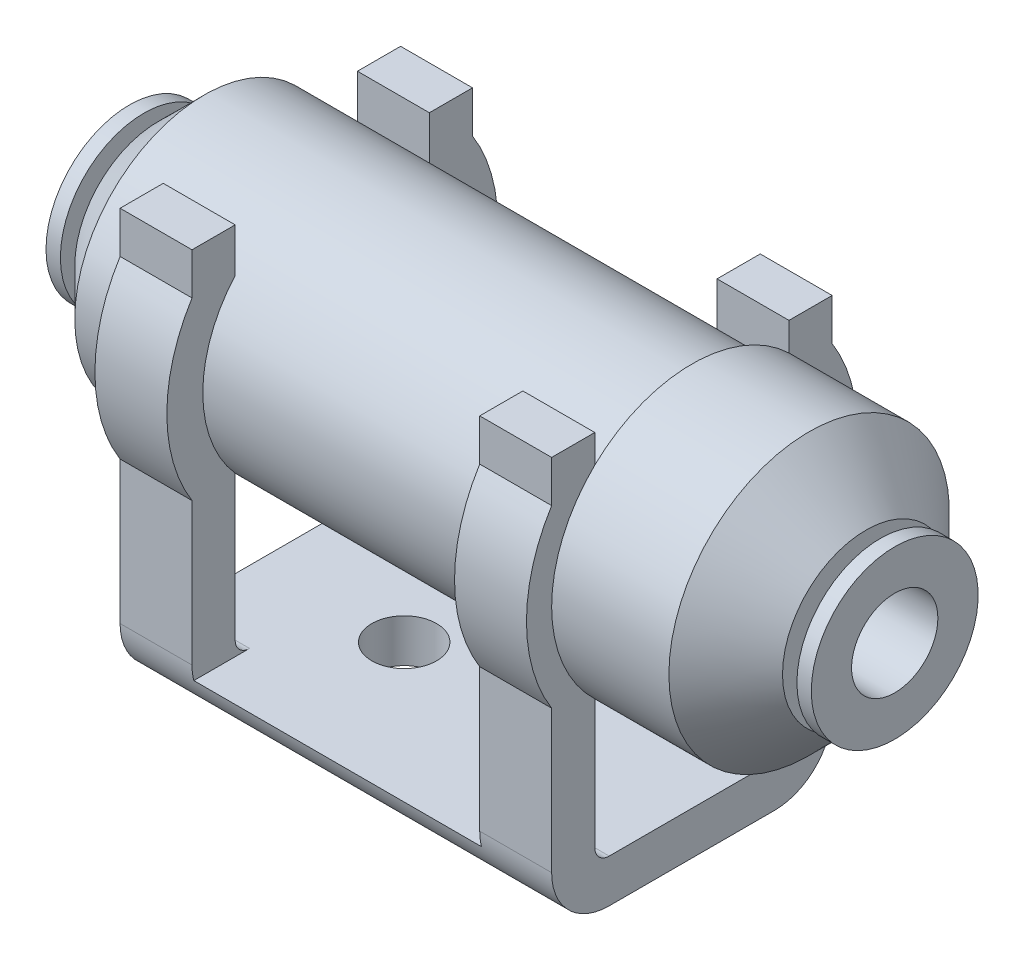
SolidWorks part; units mm, degrees
ref_plane "前视基准面" through (0, 0, 0) normal (0, 0, 1) x (1, 0, 0)
ref_plane "上视基准面" through (0, 0, 0) normal (0, 1, 0) x (1, 0, 0)
ref_plane "右视基准面" through (0, 0, 0) normal (1, 0, 0) x (0, 0, -1)
sketch "草图1" plane through (0, 0, 0) normal (0, 0, 1) x (1, 0, 0)
  line L0 (-19.1, 20) -> (-19.1, 25.8)
  line L1 (-19.1, 25.8) -> (-18.1, 25.8)
  line L2 (-18.1, 25.8) -> (-18.1, 24)
  line L3 (-18.1, 24) -> (-17.1, 24)
  line L4 (-17.1, 24) -> (-17.1, 25.8)
  line L5 (-17.1, 25.8) -> (-13.9, 29)
  line L6 (-13.9, 29) -> (20, 29)
  line L7 (20, 29) -> (20, 29.75)
  line L8 (20, 29.75) -> (28.15, 29.75)
  line L9 (28.15, 29.75) -> (32.1, 25.8)
  line L10 (32.1, 25.8) -> (32.1, 24)
  line L11 (32.1, 24) -> (33.1, 24)
  line L12 (33.1, 24) -> (33.1, 25.8)
  line L13 (33.1, 25.8) -> (34.1, 25.8)
  line L14 (34.1, 25.8) -> (34.1, 20)
  line L15 (34.1, 20) -> (-19.1, 20)
  line L16 (34.1, 20) -> (-19.1, 20) construction
revolve "旋转1" add sketch "草图1" angle 360 about L16
ref_plane "基准面4" through (-10, 0, 0) normal (1, 0, 0) x (0, 0, -1)
sketch "草图2" plane through (-10, 0, 0) normal (1, 0, 0) x (0, 0, -1)
  line L0 (-9.75, 13.9018) -> (-9.75, 4)
  line L1 (-5.75, 0) -> (5.75, 0)
  line L2 (9.75, 4) -> (9.75, 13.9018)
  line L3 (9.75, 26.0982) -> (9.75, 29)
  line L4 (9.75, 29) -> (6.75, 29)
  line L5 (6.75, 29) -> (6.75, 22)
  line L6 (6.75, 22) -> (-6.75, 22)
  line L7 (-6.75, 22) -> (-6.75, 29)
  line L8 (-6.75, 29) -> (-9.75, 29)
  line L9 (-9.75, 29) -> (-9.75, 26.0982)
  line L10 (-5.75, 3) -> (5.75, 3)
  line L11 (6.75, 4) -> (6.75, 20)
  line L12 (6.75, 20) -> (-6.75, 20)
  line L13 (-6.75, 20) -> (-6.75, 4)
  arc A0 (-9.75, 26.0982) -> (-9.75, 13.9018) centre (0, 20) ccw
  arc A1 (-9.75, 4) -> (-5.75, 0) centre (-5.75, 4) ccw
  arc A2 (5.75, 0) -> (9.75, 4) centre (5.75, 4) ccw
  arc A3 (9.75, 13.9018) -> (9.75, 26.0982) centre (0, 20) ccw
  arc A4 (-6.75, 4) -> (-5.75, 3) centre (-5.75, 4) ccw
  arc A5 (5.75, 3) -> (6.75, 4) centre (5.75, 4) ccw
extrude "凸台-拉伸1" add sketch "草图2" along normal blind 5
ref_plane "基准面5" through (20, 0, 0) normal (1, 0, 0) x (0, 0, -1)
sketch "草图3" plane through (20, 0, 0) normal (1, 0, 0) x (0, 0, -1)
  line L0 (-9.75, 13.9018) -> (-9.75, 4)
  line L1 (-5.75, 0) -> (5.75, 0)
  line L2 (9.75, 4) -> (9.75, 13.9018)
  line L3 (9.75, 26.0982) -> (9.75, 29)
  line L4 (9.75, 29) -> (6.75, 29)
  line L5 (6.75, 29) -> (6.75, 22)
  line L6 (6.75, 22) -> (-6.75, 22)
  line L7 (-6.75, 22) -> (-6.75, 29)
  line L8 (-6.75, 29) -> (-9.75, 29)
  line L9 (-9.75, 29) -> (-9.75, 26.0982)
  line L10 (-5.75, 3) -> (5.75, 3)
  line L11 (6.75, 4) -> (6.75, 20)
  line L12 (6.75, 20) -> (-6.75, 20)
  line L13 (-6.75, 20) -> (-6.75, 4)
  arc A0 (-9.75, 26.0982) -> (-9.75, 13.9018) centre (0, 20) ccw
  arc A1 (-9.75, 4) -> (-5.75, 0) centre (-5.75, 4) ccw
  arc A2 (5.75, 0) -> (9.75, 4) centre (5.75, 4) ccw
  arc A3 (9.75, 13.9018) -> (9.75, 26.0982) centre (0, 20) ccw
  arc A4 (-6.75, 4) -> (-5.75, 3) centre (-5.75, 4) ccw
  arc A5 (5.75, 3) -> (6.75, 4) centre (5.75, 4) ccw
extrude "凸台-拉伸2" add sketch "草图3" against normal blind 5
sketch "草图4" plane through (0, 0, 0) normal (1, 0, 0) x (0, 0, -1)
  line L0 (-5.75, 0) -> (5.75, 0)
  line L1 (9.623, 3) -> (-9.623, 3)
  arc A0 (-9.623, 3) -> (-5.75, 0) centre (-5.75, 4) ccw
  arc A1 (5.75, 0) -> (9.623, 3) centre (5.75, 4) ccw
sketch "草图5" plane through (0, 0, 0) normal (1, 0, 0) x (0, 0, -1)
  line L0 (-5.75, 0) -> (5.75, 0)
  line L1 (9.623, 3) -> (-9.623, 3)
  arc A0 (-9.623, 3) -> (-5.75, 0) centre (-5.75, 4) ccw
  arc A1 (5.75, 0) -> (9.623, 3) centre (5.75, 4) ccw
extrude "凸台-拉伸3" add sketch "草图4" along normal blind 15
extrude "凸台-拉伸4" add sketch "草图5" against normal blind 5
sketch "草图6" plane through (0, 0, 0) normal (0, 1, 0) x (1, 0, 0)
  circle A0 centre (0, 0) radius 2.25
extrude "切除-拉伸1" cut sketch "草图6" along normal blind 4
sketch "草图7" plane through (0, 0, 0) normal (0, 1, 0) x (1, 0, 0)
  circle A0 centre (10, 0) radius 2.25
extrude "切除-拉伸2" cut sketch "草图7" along normal blind 4
sketch "草图8" plane through (34.1, 0, 0) normal (1, 0, 0) x (0, 0, -1)
  circle A0 centre (0, 20) radius 3
extrude "切除-拉伸3" cut sketch "草图8" against normal blind 24.1
sketch "草图9" plane through (-19.1, 0, 0) normal (-1, 0, 0) x (0, 0, 1)
  circle A0 centre (0, 20) radius 3
extrude "切除-拉伸4" cut sketch "草图9" against normal blind 19.1
